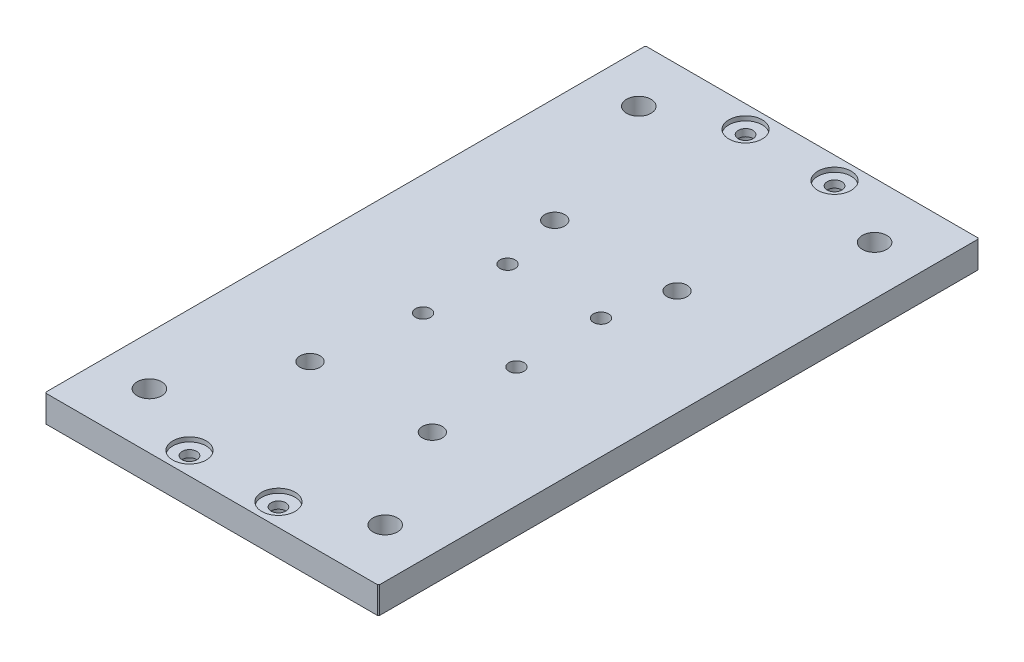
SolidWorks part; units mm, degrees
material "AL6061"
ref_plane "Front Plane" through (0, 0, 0) normal (0, 0, 1) x (1, 0, 0)
ref_plane "Top Plane" through (0, 0, 0) normal (0, 1, 0) x (1, 0, 0)
ref_plane "Right Plane" through (0, 0, 0) normal (1, 0, 0) x (0, 0, -1)
sketch "Sketch1" plane through (0, 0, 0) normal (0, 1, 0) x (1, 0, 0)
  line L1 (-75, -135) -> (75, -135)
  line L2 (-75, -135) -> (-75, 135)
  line L3 (-75, 135) -> (75, 135)
  line L4 (75, -135) -> (75, 135)
  line L5 (-75, -135) -> (75, 135) construction
  line L6 (-75, 135) -> (75, -135) construction
  point P0 (0, 0)
  dimension "D1" = 150
  dimension "D2" = 270
extrude "Boss-Extrude1" add sketch "Sketch1" along normal mid plane 12
sketch "Sketch2" plane through (0, -6, 0) normal (0, -1, 0) x (1, 0, 0)
  line L0 (0, 0) -> (0, 143.5901) construction
  line L1 (0, 0) -> (-112.2948, 0) construction
  circle A0 centre (-53, 110) radius 10
  circle A1 centre (53, 110) radius 10
  circle A2 centre (53, -110) radius 10
  circle A3 centre (-53, -110) radius 10
  dimension "D1" = 20
  dimension "D2" = 106
  dimension "D3" = 220
extrude "Cut-Extrude1" cut sketch "Sketch2" against normal blind 2
hole_wizard "M10 Clearance Hole1" positions "Sketch3" profile "Sketch4" hole size "M10" standard "GB" end condition through all
sketch "Sketch3" plane through (0, 6, 0) normal (0, 1, 0) x (1, 0, 0)
  point P0 (-53, 110)
  point P3 (53, 110)
  point P6 (-53, -110)
  point P9 (53, -110)
sketch "Sketch4" plane through (-53, 6, -110) normal (1, 0, 0) x (0, 0, 1)
  line L0 (0, 0) -> (0, 12)
  line L1 (0, 12) -> (5.5, 12)
  line L2 (5.5, 12) -> (5.5, 0)
  line L5 (5.5, 0) -> (0, 0)
  line L11 (0, -6.35) -> (0, 107.95) construction
  dimension "通孔孔直径" = 11
  dimension "通孔孔深度" = 12
sketch "Sketch5" plane through (0, 6, 0) normal (0, 1, 0) x (1, 0, 0)
  line L0 (0, 0) -> (0, 149.573) construction
  line L1 (0, 0) -> (-119.3708, 0) construction
  circle A0 centre (-20, 125) radius 7.5
  circle A1 centre (20, 125) radius 7.5
  circle A2 centre (20, -125) radius 7.5
  circle A3 centre (-20, -125) radius 7.5
  dimension "D1" = 40
  dimension "D2" = 250
  dimension "D3" = 15
extrude "Cut-Extrude2" cut sketch "Sketch5" against normal blind 2
hole_wizard "M8 Tapped Hole1" positions "Sketch6" profile "Sketch7" tap size "M8" standard "GB"
sketch "Sketch6" plane through (0, 6, 0) normal (0, 1, 0) x (1, 0, 0)
  line L0 (0, 0) -> (0, 161.6539) construction
  line L3 (0, 0) -> (-167.982, 0) construction
  line L6 (-55.5, 156.2708) -> (-55.5, -203.8551) construction
  point P19 (-55.5, 62.5)
  point P21 (-55.5, 42.5)
  point P23 (-55.5, 82.5)
  point P26 (55.5, 82.5)
  point P27 (55.5, 42.5)
  point P28 (55.5, 62.5)
  point P29 (55.5, -62.5)
  point P30 (55.5, -42.5)
  point P31 (55.5, -82.5)
  point P32 (-55.5, -82.5)
  point P33 (-55.5, -42.5)
  point P34 (-55.5, -62.5)
  dimension "D1" = 20
  dimension "D2" = 20
  dimension "D3" = 125
  dimension "D4" = 111
sketch "Sketch7" plane through (-55.5, 6, 62.5) normal (1, 0, 0) x (0, 0, 1)
  line L0 (0, 0) -> (0, 12)
  line L1 (0, 12) -> (3.4, 12)
  line L2 (3.4, 12) -> (3.4, 0)
  line L5 (3.4, 0) -> (0, 0)
  line L11 (0, -6.35) -> (0, 107.95) construction
  dimension "通孔螺纹孔钻头直径" = 6.8
  dimension "通孔螺纹孔钻头深度" = 12
cosmetic thread "Cosmetic thread 1" [suppressed] parameters "D2"=8
cosmetic thread "Cosmetic thread 2" [suppressed] parameters "D2"=8
cosmetic thread "Cosmetic thread 3" [suppressed] parameters "D2"=8
cosmetic thread "Cosmetic thread 4" [suppressed] parameters "D2"=8
cosmetic thread "Cosmetic thread 5" [suppressed] parameters "D2"=8
cosmetic thread "Cosmetic thread 6" [suppressed] parameters "D2"=8
cosmetic thread "Cosmetic thread 7" [suppressed] parameters "D2"=8
cosmetic thread "Cosmetic thread 8" [suppressed] parameters "D2"=8
cosmetic thread "Cosmetic thread 9" [suppressed] parameters "D2"=8
cosmetic thread "Cosmetic thread 10" [suppressed] parameters "D2"=8
cosmetic thread "Cosmetic thread 11" [suppressed] parameters "D2"=8
cosmetic thread "Cosmetic thread 12" [suppressed] parameters "D2"=8
hole_wizard "Hole size per socket head cap screw type 1" positions "Sketch8" profile "Sketch9" counterbore size "M6" standard "GB" end condition through all
sketch "Sketch8" plane through (0, -6, 0) normal (0, -1, 0) x (-1, 0, 0)
  point P0 (20, -125)
  point P3 (-20, -125)
  point P6 (20, 125)
  point P9 (-20, 125)
sketch "Sketch9" plane through (-20, -6, 125) normal (1, 0, 0) x (0, 0, -1)
  line L0 (0, 0) -> (0, 12)
  line L1 (0, 12) -> (3.3, 12)
  line L3 (3.3, 12) -> (3.3, 6.8)
  line L4 (3.3, 6.8) -> (5.5, 6.8)
  line L5 (5.5, 6.8) -> (5.5, 0)
  line L7 (5.5, 0) -> (0, 0)
  line L11 (0, -6.35) -> (0, 107.95) construction
  dimension "通孔孔直径" = 6.6
  dimension "通孔孔深度" = 12
  dimension "柱形沉头孔直径" = 11
  dimension "柱形沉头孔深度" = 6.8
hole_wizard "M8 Tapped Hole2" positions "Sketch10" profile "Sketch11" tap size "M8" standard "GB" end condition through all
sketch "Sketch10" plane through (0, -6, 0) normal (0, -1, 0) x (-1, 0, 0)
  line L7 (0, 0) -> (0, -70.8315) construction
  line L10 (0, 0) -> (121.8876, 0) construction
  point P106 (21, -19)
  point P109 (-21, -19)
  point P110 (-21, 19)
  point P111 (21, 19)
  dimension "D1" = 42
  dimension "D2" = 38
sketch "Sketch11" plane through (-21, -6, -19) normal (1, 0, 0) x (0, 0, -1)
  line L0 (0, 0) -> (0, 12)
  line L1 (0, 12) -> (3.4, 12)
  line L2 (3.4, 12) -> (3.4, 0)
  line L5 (3.4, 0) -> (0, 0)
  line L11 (0, -6.35) -> (0, 107.95) construction
  dimension "通孔螺纹孔钻头直径" = 6.8
  dimension "通孔螺纹孔钻头深度" = 12
cosmetic thread "Cosmetic thread 13" parameters "D2"=8
cosmetic thread "Cosmetic thread 14" parameters "D2"=8
cosmetic thread "Cosmetic thread 15" parameters "D2"=8
cosmetic thread "Cosmetic thread 16" parameters "D2"=8
chamfer "Chamfer1" distance 0.5 angle 45 4 edges at (-75, 0, 135) (75, 0, 135) (75, 0, -135) (-75, 0, -135)
hole_wizard "M8 Clearance Hole1" positions "Sketch12" profile "Sketch13" hole size "M8" standard "GB" end condition through all
sketch "Sketch12" plane through (0, 6, 0) normal (0, 1, 0) x (1, 0, 0)
  line L0 (0, 0) -> (0, -179.0562) construction
  line L4 (-27.5, 46.7) -> (27.5, 46.7)
  line L5 (-27.5, 46.7) -> (-27.5, -63.3)
  line L6 (-27.5, -63.3) -> (27.5, -63.3)
  line L7 (27.5, 46.7) -> (27.5, -63.3)
  line L8 (-74.5, -135) -> (74.5, -135) construction
  point P7 (-27.5, 46.7)
  point P8 (27.5, -63.3)
  point P135 (-27.5, -63.3)
  point P136 (27.5, 46.7)
  dimension "D1" = 55
  dimension "D2" = 110
  dimension "D3" = 71.7
sketch "Sketch13" plane through (27.5, 6, -46.7) normal (1, 0, 0) x (0, 0, 1)
  line L0 (0, 0) -> (0, 12)
  line L1 (0, 12) -> (4.5, 12)
  line L2 (4.5, 12) -> (4.5, 0)
  line L5 (4.5, 0) -> (0, 0)
  line L11 (0, -6.35) -> (0, 107.95) construction
  dimension "通孔孔直径" = 9
  dimension "通孔孔深度" = 12
